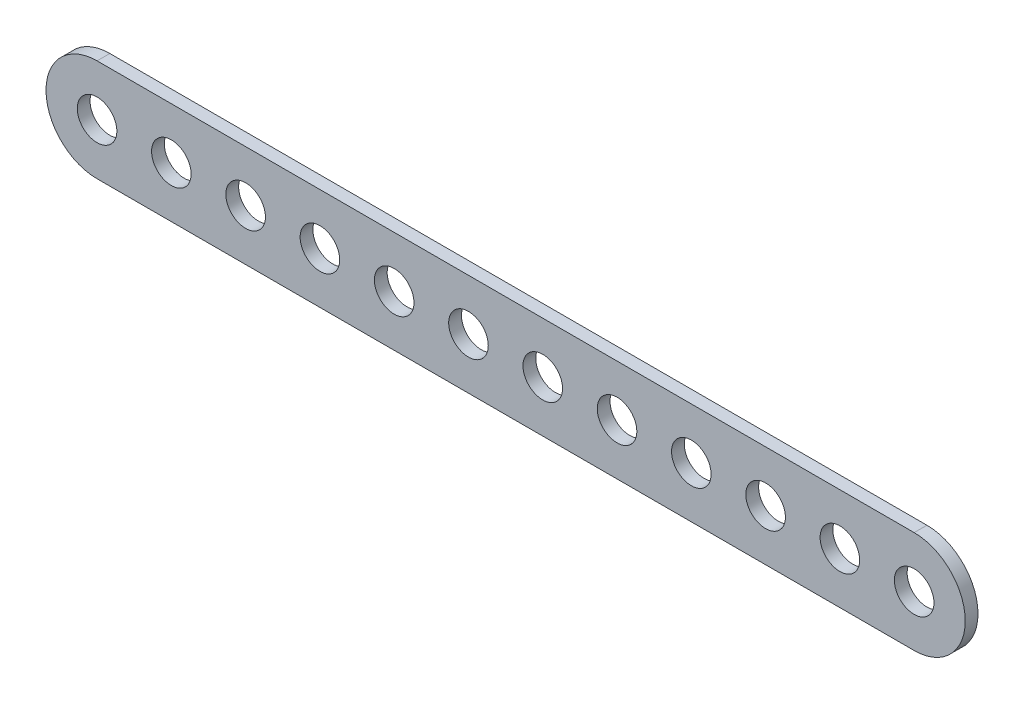
SolidWorks part; units mm, degrees
material "Thornel Mat VMA"
ref_plane "前视基准面" through (0, 0, 0) normal (0, 0, 1) x (1, 0, 0)
ref_plane "上视基准面" through (0, 0, 0) normal (0, 1, 0) x (1, 0, 0)
ref_plane "右视基准面" through (0, 0, 0) normal (1, 0, 0) x (0, 0, -1)
other "Configuration Table"
sketch "草图1" plane through (0, 0, 0) normal (0, 0, 1) x (1, 0, 0)
  line L0 (0, 0) -> (64, 0) construction
  line L1 (0, 4) -> (64, 4)
  line L2 (0, -4) -> (64, -4)
  circle A0 centre (0, 0) radius 1.55
  arc A2 (0, 4) -> (0, -4) centre (0, 0) ccw
  arc A3 (64, -4) -> (64, 4) centre (64, 0) ccw
  circle A4 centre (5.8182, 0) radius 1.55
  circle A5 centre (11.6364, 0) radius 1.55
  circle A6 centre (17.4545, 0) radius 1.55
  circle A7 centre (23.2727, 0) radius 1.55
  circle A8 centre (29.0909, 0) radius 1.55
  circle A9 centre (34.9091, 0) radius 1.55
  circle A10 centre (40.7273, 0) radius 1.55
  circle A11 centre (46.5455, 0) radius 1.55
  circle A12 centre (52.3636, 0) radius 1.55
  circle A13 centre (58.1818, 0) radius 1.55
  circle A14 centre (64, 0) radius 1.55
  point P5 (32, 0)
  point P10 (42.4601, 0)
  point P11 (64, 0)
  dimension "D1" = 3.1
  dimension "D2" = 4
  dimension "D3" = 64
  dimension "D4" = 12
extrude "凸台-拉伸1" add sketch "草图1" along normal blind 1
